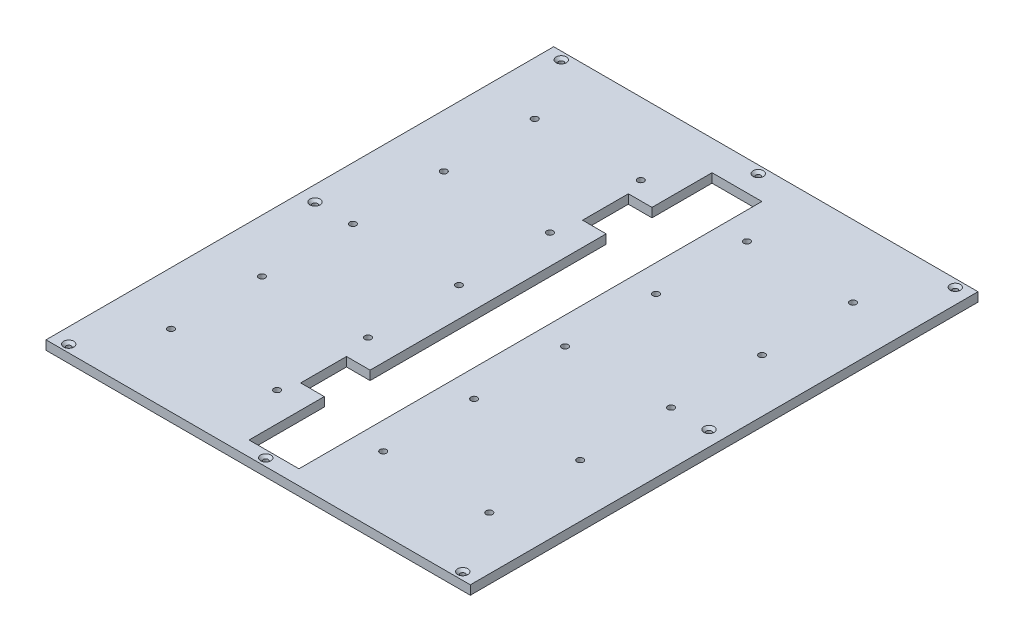
from build123d import *

# Parameters (mm, degrees)
SKETCH1_W                     = 560
SKETCH1_H                     = 670
BOSS_EXTRUDE1_DEPTH           = 12
SKETCH3_R                     = 4.25
SKETCH3_R_2                   = 0.639613625
CUT_EXTRUDE1_DEPTH            = 12
MIRROR2_COPY_1_SKETCH_R       = 4.25
MIRROR2_COPY_1_SKETCH_R_2     = 0.639613625
MIRROR2_COPY_1_DEPTH          = 12
CSK_FOR_M6_SFHCS1_D           = 6.6
CSK_FOR_M6_SFHCS1_CSINK_D     = 13.44
CSK_FOR_M6_SFHCS1_CSINK_ANGLE = 90
SKETCH10_W                    = 65.8
SKETCH10_H                    = 611
CUT_EXTRUDE2_DEPTH            = 111
SKETCH11_W                    = 31.663111861
SKETCH11_H                    = 60.455114524
CUT_EXTRUDE3_DEPTH            = 55


with BuildPart() as part:
    # Sketch1 → Boss-Extrude1 (new body)
    with BuildSketch(Plane(origin=(0, 0, 0), x_dir=(1, 0, 0), z_dir=(0, 1, 0))):
        Rectangle(SKETCH1_W, SKETCH1_H)
    extrude(amount=BOSS_EXTRUDE1_DEPTH)

    # Sketch3 → Cut-Extrude1 (cut)
    with BuildSketch(Plane(origin=(0, 12, 0), x_dir=(1, 0, 0), z_dir=(0, 1, 0))):
        with Locations(Location((210, 240, 0), (0, 0, 270))):
            Circle(SKETCH3_R)
        with Locations(Location((70, 240, 0), (0, 0, 270))):
            Circle(SKETCH3_R)
        with Locations(Location((210, 120, 0), (0, 0, 270))):
            Circle(SKETCH3_R)
        with Locations(Location((70, 120, 0), (0, 0, 270))):
            Circle(SKETCH3_R)
        with Locations(Location((70, 0, 0), (0, 0, 270))):
            Circle(SKETCH3_R)
        with Locations(Location((210, 0, 0), (0, 0, 270))):
            Circle(SKETCH3_R)
        with Locations(Location((0, 0, 0), (0, 0, 270))):
            Circle(SKETCH3_R_2)
    cut_extrude1 = extrude(amount=-CUT_EXTRUDE1_DEPTH, mode=Mode.SUBTRACT)

    # Mirror1: Cut-Extrude1 across plane
    add(cut_extrude1.mirror(Plane(origin=(0, 0, 0), x_dir=(0, 0, 1), z_dir=(1, 0, 0))), mode=Mode.SUBTRACT)

    # Mirror2: Cut-Extrude1 across plane
    add(cut_extrude1.mirror(Plane.XY), mode=Mode.SUBTRACT)

    # Mirror2 copy 1 sketch → Mirror2 copy 1 (cut)
    with BuildSketch(Plane(origin=(0, 12, 0), x_dir=(-1, 0, 0), z_dir=(0, 1, 0))):
        with Locations(Location((210, 240, 0), (0, 0, 270))):
            Circle(MIRROR2_COPY_1_SKETCH_R)
        with Locations(Location((70, 240, 0), (0, 0, 270))):
            Circle(MIRROR2_COPY_1_SKETCH_R)
        with Locations(Location((210, 120, 0), (0, 0, 270))):
            Circle(MIRROR2_COPY_1_SKETCH_R)
        with Locations(Location((70, 120, 0), (0, 0, 270))):
            Circle(MIRROR2_COPY_1_SKETCH_R)
        with Locations(Location((70, 0, 0), (0, 0, 270))):
            Circle(MIRROR2_COPY_1_SKETCH_R)
        with Locations(Location((210, 0, 0), (0, 0, 270))):
            Circle(MIRROR2_COPY_1_SKETCH_R)
        with Locations(Location((0, 0, 0), (0, 0, 270))):
            Circle(MIRROR2_COPY_1_SKETCH_R_2)
    extrude(amount=-MIRROR2_COPY_1_DEPTH, mode=Mode.SUBTRACT)

    # CSK for M6 SFHCS1 (through all)
    with Locations(Plane(origin=(0, 12, 0), x_dir=(1, 0, 0), z_dir=(0, 1, 0))):
        with Locations((0, 0), (260, 0), (0, 325), (260, 325), (0, -325), (-260, 0), (-260, 325), (-260, -325), (260, -325)):
            CounterSinkHole(CSK_FOR_M6_SFHCS1_D / 2, CSK_FOR_M6_SFHCS1_CSINK_D / 2, counter_sink_angle=CSK_FOR_M6_SFHCS1_CSINK_ANGLE)

    # Sketch10 → Cut-Extrude2 (cut)
    with BuildSketch(Plane(origin=(0, 12, 0), x_dir=(1, 0, 0), z_dir=(0, 1, 0))):
        with Locations((1.4, -10)):
            Rectangle(SKETCH10_W, SKETCH10_H)
    extrude(amount=-CUT_EXTRUDE2_DEPTH, mode=Mode.SUBTRACT)

    # Sketch11 → Cut-Extrude3 (cut)
    with BuildSketch(Plane(origin=(0, 12, 0), x_dir=(1, 0, 0), z_dir=(0, 1, 0))):
        with Locations((-46.831555931, -186)):
            Rectangle(SKETCH11_W, SKETCH11_H)
    cut_extrude3 = extrude(amount=-CUT_EXTRUDE3_DEPTH, mode=Mode.SUBTRACT)

    # Mirror3: Cut-Extrude3 across plane
    add(cut_extrude3.mirror(Plane.XY), mode=Mode.SUBTRACT)


solid = part.part
